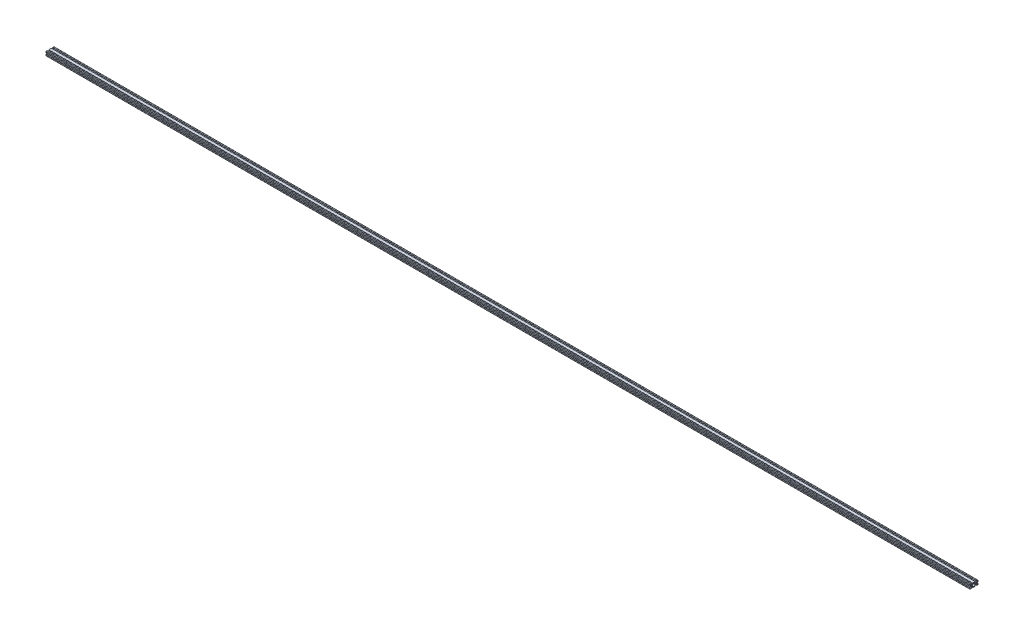
from build123d import *

# Parameters (mm, degrees)
SKETCH1_R                               = 2.5
ALUMINUM_PROFILE_20_X_40_X_R1_5_1_DEPTH = 4546
M6_TAPPED_HOLE1_D                       = 5
M6_TAPPED_HOLE1_DEPTH                   = 15
M6_TAPPED_HOLE1_TIP                     = 1.502151548


with BuildPart() as part:
    # Sketch1 → Aluminum profile 20 X 40 X R1.5(1) (new body)
    with BuildSketch(Plane(origin=(-2530.155642023, -1602.186915496, 0), x_dir=(0, 1, 0), z_dir=(1, 0, 0))):
        with BuildLine():
            Line((-3.6, 10), (-3.6, 9.5))
            Line((-3.6, 9.5), (-3.1, 9.5))
            Line((-3.1, 9.5), (-3.1, 8.5))
            Line((-3.1, 8.5), (-5.5, 8.5))
            Line((-5.5, 8.5), (-5.5, 6.65))
            Line((-5.5, 6.65), (-2.75, 3.9))
            Line((-2.75, 3.9), (2.75, 3.9))
            Line((2.75, 3.9), (5.5, 6.65))
            Line((5.5, 6.65), (5.5, 8.5))
            Line((5.5, 8.5), (3.1, 8.5))
            Line((3.1, 8.5), (3.1, 9.5))
            Line((3.1, 9.5), (3.6, 9.5))
            Line((3.6, 9.5), (3.6, 10))
            Line((3.6, 10), (8.5, 10))
            ThreePointArc((8.5, 10), (9.560660172, 9.560660172), (10, 8.5))
            Line((10, 8.5), (10, 3.6))
            Line((10, 3.6), (9.5, 3.6))
            Line((9.5, 3.6), (9.5, 3.1))
            Line((9.5, 3.1), (8.5, 3.1))
            Line((8.5, 3.1), (8.5, 5.5))
            Line((8.5, 5.5), (6.65, 5.5))
            Line((6.65, 5.5), (3.9, 2.75))
            Line((3.9, 2.75), (3.9, -2.75))
            Line((3.9, -2.75), (6.65, -5.5))
            Line((6.65, -5.5), (8.5, -5.5))
            Line((8.5, -5.5), (8.5, -3.1))
            Line((8.5, -3.1), (9.5, -3.1))
            Line((9.5, -3.1), (9.5, -3.6))
            Line((9.5, -3.6), (10, -3.6))
            Line((10, -3.6), (10, -16.4))
            Line((10, -16.4), (9.5, -16.4))
            Line((9.5, -16.4), (9.5, -16.9))
            Line((9.5, -16.9), (8.5, -16.9))
            Line((8.5, -16.9), (8.5, -14.5))
            Line((8.5, -14.5), (6.65, -14.5))
            Line((6.65, -14.5), (3.9, -17.25))
            Line((3.9, -17.25), (3.9, -22.75))
            Line((3.9, -22.75), (6.65, -25.5))
            Line((6.65, -25.5), (8.5, -25.5))
            Line((8.5, -25.5), (8.5, -23.1))
            Line((8.5, -23.1), (9.5, -23.1))
            Line((9.5, -23.1), (9.5, -23.6))
            Line((9.5, -23.6), (10, -23.6))
            Line((10, -23.6), (10, -28.5))
            ThreePointArc((10, -28.5), (9.560660172, -29.560660172), (8.5, -30))
            Line((8.5, -30), (3.6, -30))
            Line((3.6, -30), (3.6, -29.5))
            Line((3.6, -29.5), (3.1, -29.5))
            Line((3.1, -29.5), (3.1, -28.5))
            Line((3.1, -28.5), (5.5, -28.5))
            Line((5.5, -28.5), (5.5, -26.65))
            Line((5.5, -26.65), (2.75, -23.9))
            Line((2.75, -23.9), (-2.75, -23.9))
            Line((-2.75, -23.9), (-5.5, -26.65))
            Line((-5.5, -26.65), (-5.5, -28.5))
            Line((-5.5, -28.5), (-3.1, -28.5))
            Line((-3.1, -28.5), (-3.1, -29.5))
            Line((-3.1, -29.5), (-3.6, -29.5))
            Line((-3.6, -29.5), (-3.6, -30))
            Line((-3.6, -30), (-8.5, -30))
            ThreePointArc((-8.5, -30), (-9.560660172, -29.560660172), (-10, -28.5))
            Line((-10, -28.5), (-10, -23.6))
            Line((-10, -23.6), (-9.5, -23.6))
            Line((-9.5, -23.6), (-9.5, -23.1))
            Line((-9.5, -23.1), (-8.5, -23.1))
            Line((-8.5, -23.1), (-8.5, -25.5))
            Line((-8.5, -25.5), (-6.65, -25.5))
            Line((-6.65, -25.5), (-3.9, -22.75))
            Line((-3.9, -22.75), (-3.9, -17.25))
            Line((-3.9, -17.25), (-6.65, -14.5))
            Line((-6.65, -14.5), (-8.5, -14.5))
            Line((-8.5, -14.5), (-8.5, -16.9))
            Line((-8.5, -16.9), (-9.5, -16.9))
            Line((-9.5, -16.9), (-9.5, -16.4))
            Line((-9.5, -16.4), (-10, -16.4))
            Line((-10, -16.4), (-10, -3.6))
            Line((-10, -3.6), (-9.5, -3.6))
            Line((-9.5, -3.6), (-9.5, -3.1))
            Line((-9.5, -3.1), (-8.5, -3.1))
            Line((-8.5, -3.1), (-8.5, -5.5))
            Line((-8.5, -5.5), (-6.65, -5.5))
            Line((-6.65, -5.5), (-3.9, -2.75))
            Line((-3.9, -2.75), (-3.9, 2.75))
            Line((-3.9, 2.75), (-6.65, 5.5))
            Line((-6.65, 5.5), (-8.5, 5.5))
            Line((-8.5, 5.5), (-8.5, 3.1))
            Line((-8.5, 3.1), (-9.5, 3.1))
            Line((-9.5, 3.1), (-9.5, 3.6))
            Line((-9.5, 3.6), (-10, 3.6))
            Line((-10, 3.6), (-10, 8.5))
            ThreePointArc((-10, 8.5), (-9.560660172, 9.560660172), (-8.5, 10))
            Line((-8.5, 10), (-3.6, 10))
        make_face()
        Circle(SKETCH1_R, mode=Mode.SUBTRACT)
        with Locations((0, -20)):
            Circle(SKETCH1_R, mode=Mode.SUBTRACT)
        Polygon((8.85, -10), (2.75, -3.9), (-2.75, -3.9), (-8.85, -10), (-2.75, -16.1), (2.75, -16.1), align=None, mode=Mode.SUBTRACT)
    extrude(amount=ALUMINUM_PROFILE_20_X_40_X_R1_5_1_DEPTH)

    # M6 Tapped Hole1
    with Locations(Plane(origin=(2015.844357977, 0, 0), x_dir=(0, 0, -1), z_dir=(1, 0, 0))):
        with Locations((0, -1602.186915496), (20, -1602.186915496)):
            Hole(M6_TAPPED_HOLE1_D / 2, depth=M6_TAPPED_HOLE1_DEPTH)
            with Locations((0, 0, -(M6_TAPPED_HOLE1_DEPTH + M6_TAPPED_HOLE1_TIP / 2))):  # 118° drill point
                Cone(0, M6_TAPPED_HOLE1_D / 2, M6_TAPPED_HOLE1_TIP, mode=Mode.SUBTRACT)


solid = part.part
